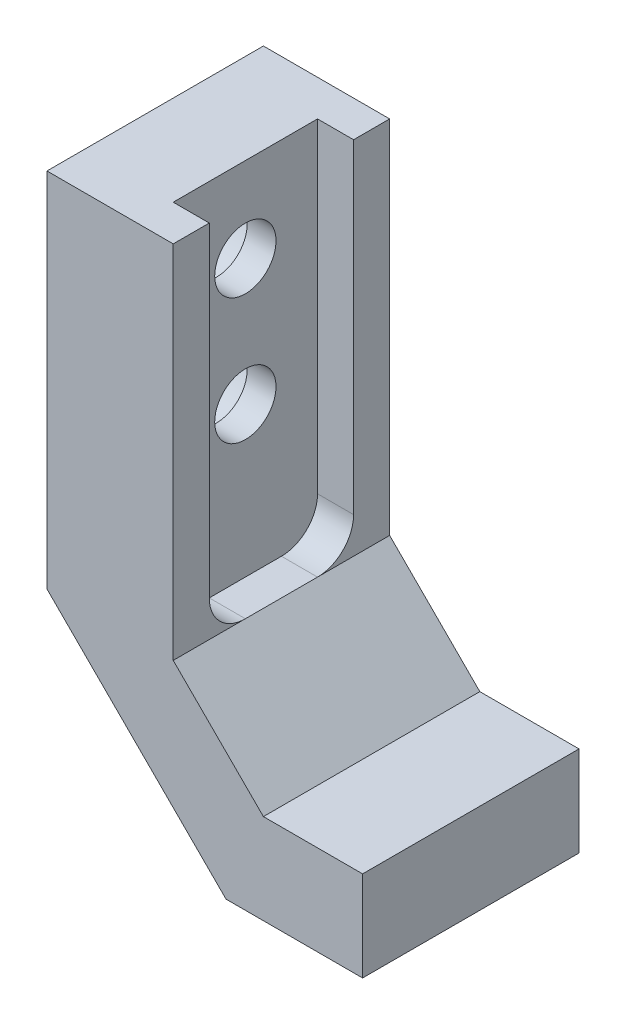
from build123d import *

# Parameters (mm, degrees)
EXTRUDE_1_DEPTH              = 6
SKETCH_2_W                   = 2
SKETCH_2_H                   = 8
CUT_EXTRUDE_1_DEPTH          = 20
FILLET_1_R                   = 2
HOLE_WIZARD_M3_1_D           = 3.4
HOLE_WIZARD_M3_1_CBORE_D     = 6
HOLE_WIZARD_M3_1_CBORE_DEPTH = 3.4


with BuildPart() as part:
    # 草图1 → 凸台-拉伸1 (new, symmetric)
    with BuildSketch(Plane.XY):
        Polygon((0, 0), (0, -20.071067812), (9.928932188, -30), (17.5, -30), (17.5, -25), (12, -25), (7, -20), (7, 0), align=None)
    extrude(amount=EXTRUDE_1_DEPTH, both=True)

    # 草图2 → 切除-拉伸1 (cut)
    with BuildSketch(Plane(origin=(0, 0, 0), x_dir=(1, 0, 0), z_dir=(0, 1, 0))):
        with Locations((6, 0)):
            Rectangle(SKETCH_2_W, SKETCH_2_H)
    extrude(amount=-CUT_EXTRUDE_1_DEPTH, mode=Mode.SUBTRACT)

    # 圆角1
    fillet_1_edges = [part.edges().sort_by_distance(p)[0] for p in [
        (6, -20, -4),
        (6, -20, 4),
    ]]
    fillet(fillet_1_edges, radius=FILLET_1_R)

    # M3 六角圆柱头螺钉的柱形沉头孔1 (through all)
    with Locations(Plane.ZY):
        with Locations((0, -4.7), (0, -11.7)):
            CounterBoreHole(HOLE_WIZARD_M3_1_D / 2, HOLE_WIZARD_M3_1_CBORE_D / 2, HOLE_WIZARD_M3_1_CBORE_DEPTH)


solid = part.part
